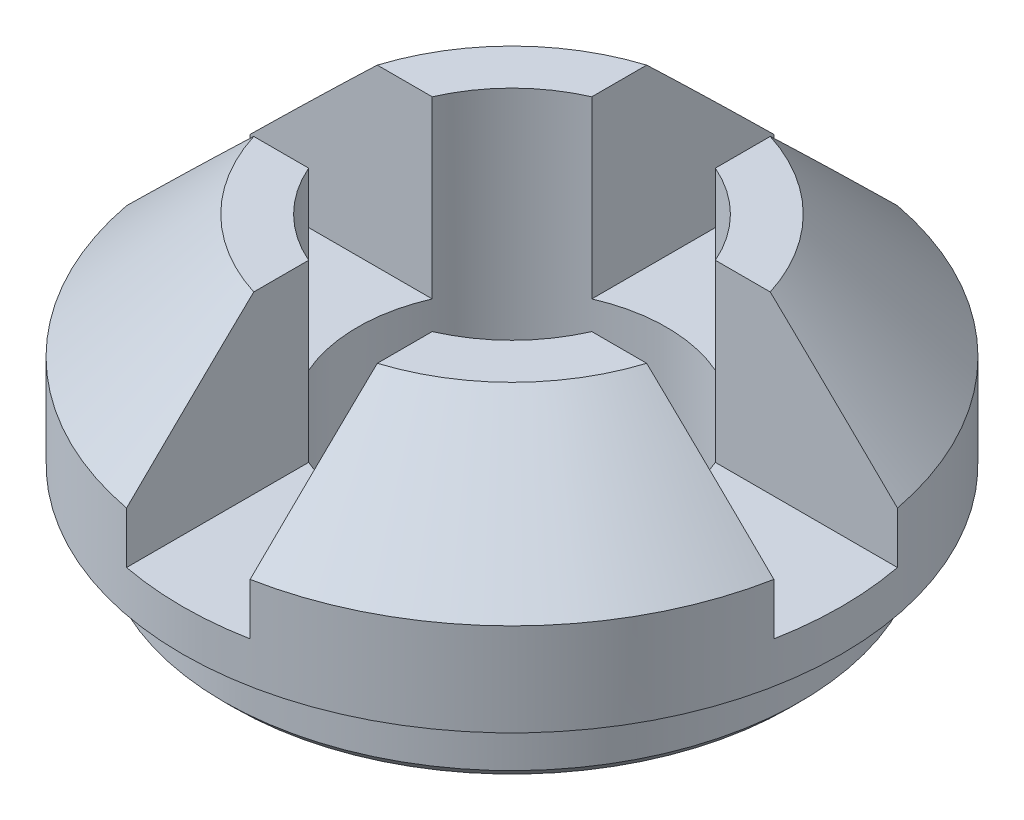
from build123d import *

# Parameters (mm, degrees)
SKETCH2_R          = 7.5
CUT_EXTRUDE1_DEPTH = 31
SKETCH3_W          = 40.68
SKETCH3_H          = 6
CUT_EXTRUDE2_DEPTH = 8.5
CIRPATTERN1_COUNT  = 4
CHAMFER1_SIZE      = 0.5
CHAMFER2_SIZE      = 0.5


with BuildPart() as part:
    # Sketch1 → Revolve1 (revolve)
    with BuildSketch(Plane.XY, mode=Mode.PRIVATE) as revolve1_sk:
        Polygon((0, 0), (-14, 0), (-14, 3.5), (-16, 3.5), (-16, 8), (-10, 14), (0, 14), align=None)
    revolve(revolve1_sk.sketch.rotate(Axis((0, 0, 0), (0, 1, 0)), 270), axis=Axis((0, 0, 0), (0, 1, 0)))

    # Sketch2 → Cut-Extrude1 (cut)
    with BuildSketch(Plane(origin=(0, 14, 0), x_dir=(1, 0, 0), z_dir=(0, 1, 0))):
        with Locations(Location((0, 0, 0), (0, 0, 270))):
            Circle(SKETCH2_R)
    extrude(amount=-CUT_EXTRUDE1_DEPTH, mode=Mode.SUBTRACT)

    # Sketch3 → Cut-Extrude2 (cut)
    with BuildSketch(Plane(origin=(0, 14, 0), x_dir=(1, 0, 0), z_dir=(0, 1, 0))):
        Rectangle(SKETCH3_W, SKETCH3_H)
    cut_extrude2 = extrude(amount=-CUT_EXTRUDE2_DEPTH, mode=Mode.SUBTRACT)

    # CirPattern1: Cut-Extrude2 ×4 about axis
    cirpattern1_axis = Axis((0, -17, 0), (0, 1, 0))
    for i in range(1, CIRPATTERN1_COUNT):
        add(cut_extrude2.rotate(cirpattern1_axis, i * 360 / CIRPATTERN1_COUNT), mode=Mode.SUBTRACT)

    # Chamfer1
    chamfer1_edges = [part.edges().sort_by_distance(p)[0] for p in [
        (0, 0, 14),
    ]]
    chamfer(chamfer1_edges, length=CHAMFER1_SIZE)

    # Chamfer2
    chamfer2_edges = [part.edges().sort_by_distance(p)[0] for p in [
        (0, 0, -7.5),
    ]]
    chamfer(chamfer2_edges, length=CHAMFER2_SIZE)


solid = part.part
